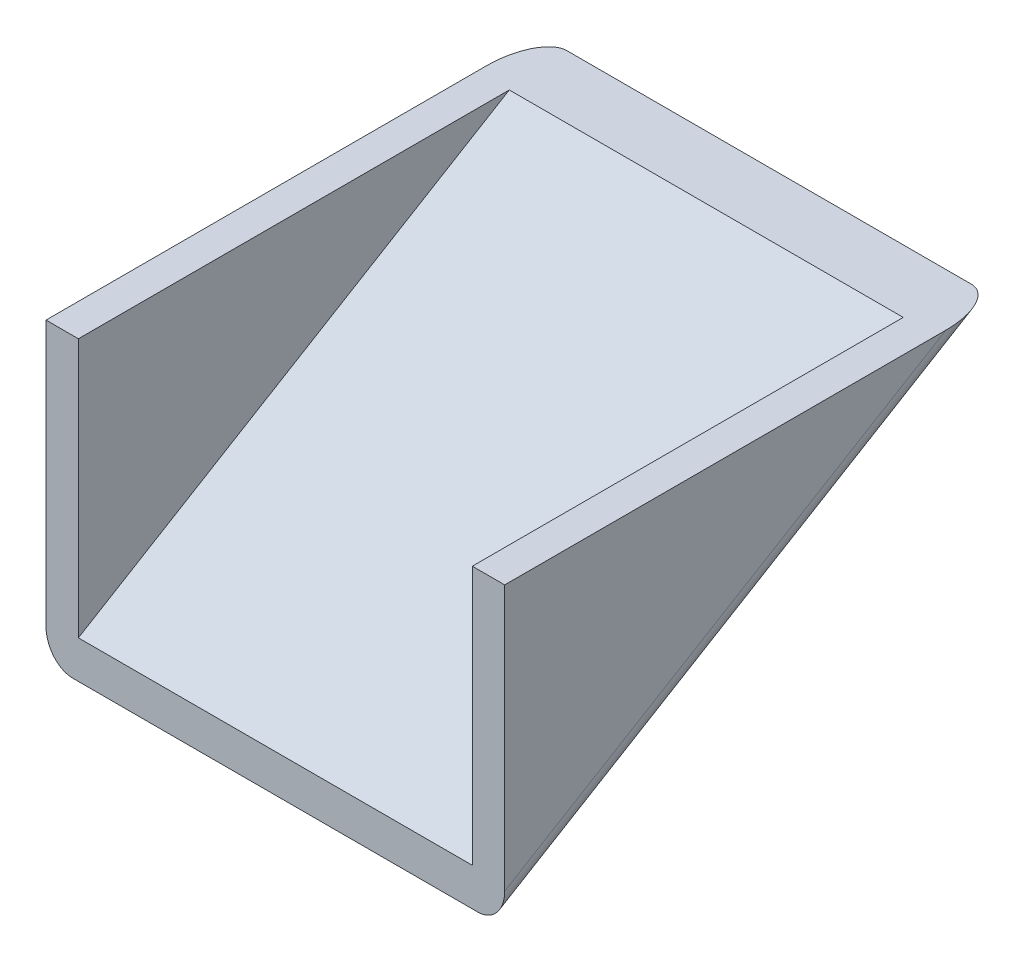
from build123d import *

# Parameters (mm, degrees)
SKETCH_2_W          = 170
SKETCH_2_H          = 110
EXTRUDE_2_DEPTH     = 500
SKETCH_5_OUTSIDE_W  = 609.888
SKETCH_5_OUTSIDE_H  = 219.888
CUT_EXTRUDE_3_DEPTH = 200
FILLET_2_R          = 10
SHELL_2_T           = -12


with BuildPart() as part:
    # 草图2 → 凸台-拉伸2 (new body)
    with BuildSketch(Plane.XY):
        Rectangle(SKETCH_2_W, SKETCH_2_H)
    extrude(amount=EXTRUDE_2_DEPTH)

    # 草图5 outside → 切除-拉伸3 (cut)
    with BuildSketch(Plane.ZY.offset(85)):
        with Locations((250, 0)):
            Rectangle(SKETCH_5_OUTSIDE_W, SKETCH_5_OUTSIDE_H)
        Polygon((386.948309985, 55), (386.948309985, -55), (203.948309985, 55), align=None, mode=Mode.SUBTRACT)
    extrude(amount=-CUT_EXTRUDE_3_DEPTH, mode=Mode.SUBTRACT)

    # 圆角2
    fillet_2_edges = [part.edges().sort_by_distance(p)[0] for p in [
        (85, 0, 295.448309985),
        (-85, 0, 295.448309985),
    ]]
    fillet(fillet_2_edges, radius=FILLET_2_R)

    # 抽壳2
    shell_2_openings = [part.faces().sort_by_distance(p)[0] for p in [
        (0, 55, 295.682357503),
        (0, 0.1406843, 386.948309985),
    ]]
    offset(amount=SHELL_2_T, openings=shell_2_openings, kind=Kind.INTERSECTION)


solid = part.part
